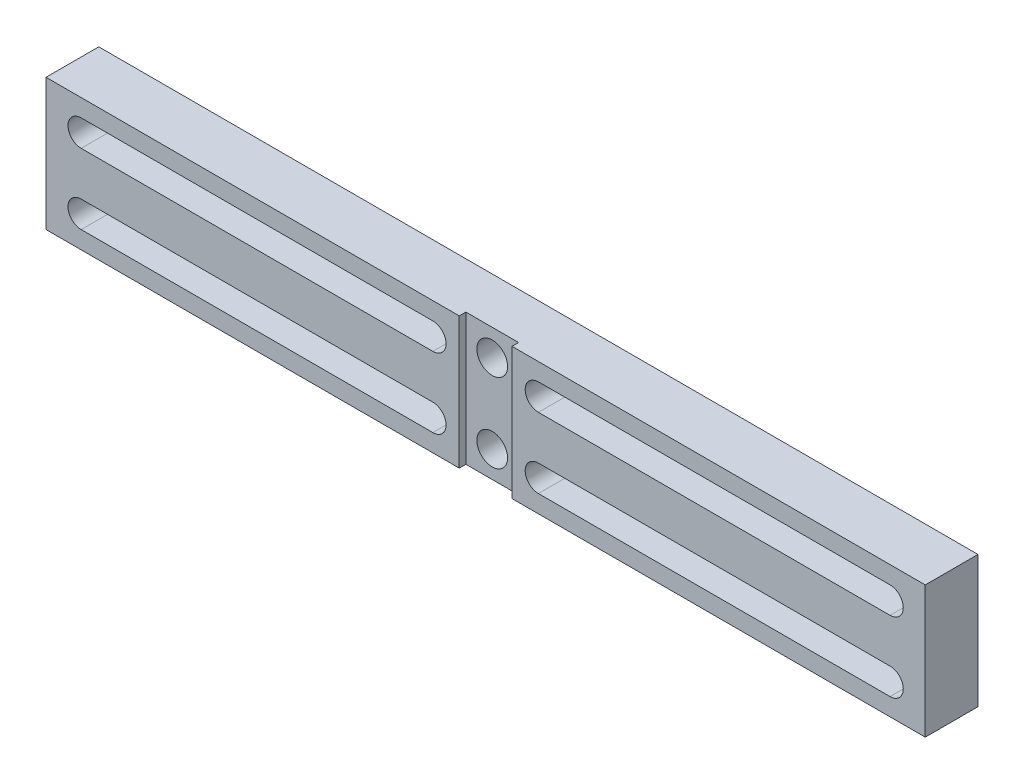
from build123d import *

# Parameters (mm, degrees)
SKETCH_1_W          = 200
SKETCH_1_H          = 30
EXTRUDE_1_DEPTH     = 12
SKETCH_2_W          = 12
SKETCH_2_H          = 30
CUT_EXTRUDE_1_DEPTH = 1.5
CUT_EXTRUDE_2_REACH = 103.662
SKETCH_3_R          = 3.5


with BuildPart() as part:
    # 草图1 → 凸台-拉伸1 (new body)
    with BuildSketch(Plane.XY):
        Rectangle(SKETCH_1_W, SKETCH_1_H)
        with BuildLine():
            Line((-92, 11), (-12, 11))
            ThreePointArc((-12, 11), (-9, 8), (-12, 5))
            Line((-12, 5), (-92, 5))
            ThreePointArc((-92, 5), (-95, 8), (-92, 11))
        make_face(mode=Mode.SUBTRACT)
        with BuildLine():
            Line((-92, -11), (-12, -11))
            ThreePointArc((-12, -11), (-9, -8), (-12, -5))
            Line((-12, -5), (-92, -5))
            ThreePointArc((-92, -5), (-95, -8), (-92, -11))
        make_face(mode=Mode.SUBTRACT)
        with BuildLine():
            Line((92, 11), (12, 11))
            ThreePointArc((12, 11), (9, 8), (12, 5))
            Line((12, 5), (92, 5))
            ThreePointArc((92, 5), (95, 8), (92, 11))
        make_face(mode=Mode.SUBTRACT)
        with BuildLine():
            Line((92, -11), (12, -11))
            ThreePointArc((12, -11), (9, -8), (12, -5))
            Line((12, -5), (92, -5))
            ThreePointArc((92, -5), (95, -8), (92, -11))
        make_face(mode=Mode.SUBTRACT)
    extrude(amount=EXTRUDE_1_DEPTH)

    # 草图2 → 切除-拉伸1 (cut)
    with BuildSketch(Plane.XY.offset(12)):
        Rectangle(SKETCH_2_W, SKETCH_2_H)
    extrude(amount=-CUT_EXTRUDE_1_DEPTH, mode=Mode.SUBTRACT)

    # 草图3 → 切除-拉伸2 (cut, up to next)
    with BuildSketch(Plane.XY.offset(10.5), mode=Mode.PRIVATE) as cut_extrude_2_sk1:
        with Locations((0, 9)):
            Circle(SKETCH_3_R)
    cut_extrude_2_tool1 = extrude(cut_extrude_2_sk1.sketch, amount=-CUT_EXTRUDE_2_REACH, mode=Mode.PRIVATE) & part.part
    # 草图3 → 切除-拉伸2 (cut, up to next)
    with BuildSketch(Plane.XY.offset(10.5), mode=Mode.PRIVATE) as cut_extrude_2_sk2:
        with Locations((0, -9)):
            Circle(SKETCH_3_R)
    cut_extrude_2_tool2 = extrude(cut_extrude_2_sk2.sketch, amount=-CUT_EXTRUDE_2_REACH, mode=Mode.PRIVATE) & part.part
    add(cut_extrude_2_tool1.solids().sort_by_distance((0, 9, 10.5))[0], mode=Mode.SUBTRACT)
    add(cut_extrude_2_tool2.solids().sort_by_distance((0, -9, 10.5))[0], mode=Mode.SUBTRACT)


solid = part.part
